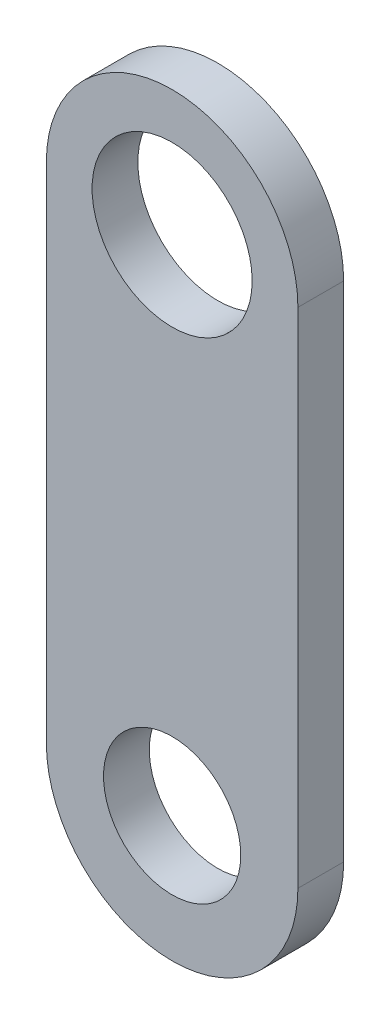
from build123d import *

# Parameters (mm, degrees)
SKETCH1_R           = 15
SKETCH1_R_2         = 17.5
BOSS_EXTRUDE1_DEPTH = 10


with BuildPart() as part:
    # Sketch1 → Boss-Extrude1 (new body)
    with BuildSketch(Plane.XY):
        with BuildLine():
            Line((-27.5, 110), (-27.5, 0))
            ThreePointArc((-27.5, 0), (0, -27.5), (27.5, 0))
            Line((27.5, 0), (27.5, 110))
            ThreePointArc((27.5, 110), (0, 137.5), (-27.5, 110))
        make_face()
        Circle(SKETCH1_R, mode=Mode.SUBTRACT)
        with Locations((0, 110)):
            Circle(SKETCH1_R_2, mode=Mode.SUBTRACT)
    extrude(amount=BOSS_EXTRUDE1_DEPTH)


solid = part.part
